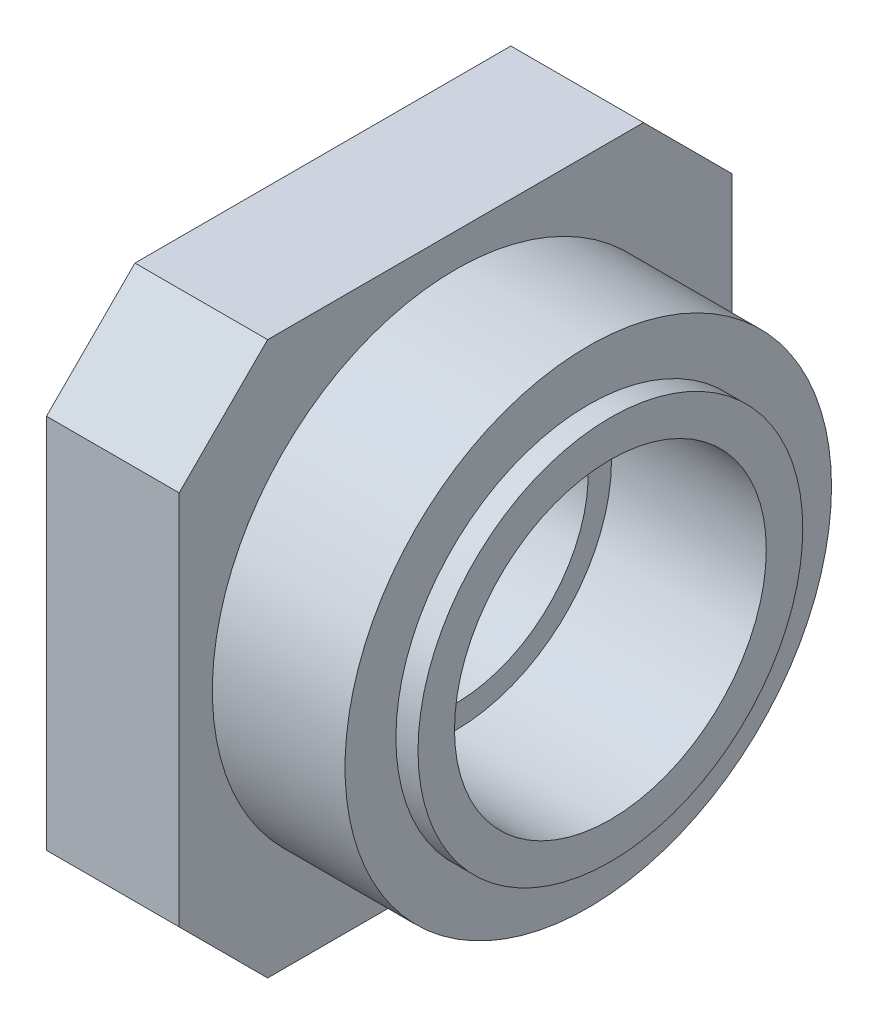
SolidWorks part; units mm, degrees
ref_plane "Front Plane" through (0, 0, 0) normal (0, 0, 1) x (1, 0, 0)
ref_plane "Top Plane" through (0, 0, 0) normal (0, 1, 0) x (1, 0, 0)
ref_plane "Right Plane" through (0, 0, 0) normal (1, 0, 0) x (0, 0, -1)
sketch "Sketch1" plane through (0, 0, 0) normal (1, 0, 0) x (0, 0, -1)
  line L1 (-12.5, -12.5) -> (12.5, -12.5)
  line L2 (-12.5, -12.5) -> (-12.5, 12.5)
  line L3 (-12.5, 12.5) -> (12.5, 12.5)
  line L4 (12.5, -12.5) -> (12.5, 12.5)
  line L5 (-12.5, -12.5) -> (12.5, 12.5) construction
  line L6 (-12.5, 12.5) -> (12.5, -12.5) construction
  point P0 (0, 0)
  dimension "D1" = 25
extrude "Boss-Extrude1" add sketch "Sketch1" along normal mid plane 6
hole_wizard "M14 Tapped Hole1" positions "Sketch3" profile "Sketch4" tap size "M14" standard "ISO"
sketch "Sketch3" plane through (-3, 0, 0) normal (-1, 0, 0) x (0, 0, 1)
  point P0 (0, 0)
sketch "Sketch4" plane through (-3, 0, 0) normal (0, 1, 0) x (0, 0, 1)
  line L0 (0, 0) -> (0, 37.6052)
  line L1 (0, 37.6052) -> (6, 34)
  line L2 (6, 34) -> (6, 0)
  line L5 (6, 0) -> (0, 0)
  line L10 (0, 37.6052) -> (-6, 34) construction
  line L11 (0, -6.35) -> (0, 107.95) construction
  dimension "螺纹孔钻头直径" = 12
  dimension "螺纹孔钻头深度" = 34
  dimension "导头角度" = 118
cosmetic thread "Cosmetic Thread1" parameters "D1"=28, "D2"=14
sketch "Sketch5" plane through (3, 0, 0) normal (1, 0, 0) x (0, 0, -1)
  circle A0 centre (0, 0) radius 11
  circle A1 centre (0, 0) radius 7.05
  dimension "D1" = 14.1
  dimension "D2" = 22
extrude "Boss-Extrude2" add sketch "Sketch5" along normal blind 7
sketch "Sketch6" plane through (10, 0, 0) normal (1, 0, 0) x (0, 0, -1)
  circle A0 centre (0, 0) radius 8.7
  circle A1 centre (0, 0) radius 11
  circle A2 centre (0, 0) radius 11 construction
  dimension "D1" = 17.4
extrude "Cut-Extrude1" cut sketch "Sketch6" against normal blind 1
chamfer "Chamfer1" distance 4 angle 45 4 edges at (0, -12.5, 12.5) (0, -12.5, -12.5) (0, 12.5, -12.5) (0, 12.5, 12.5)
